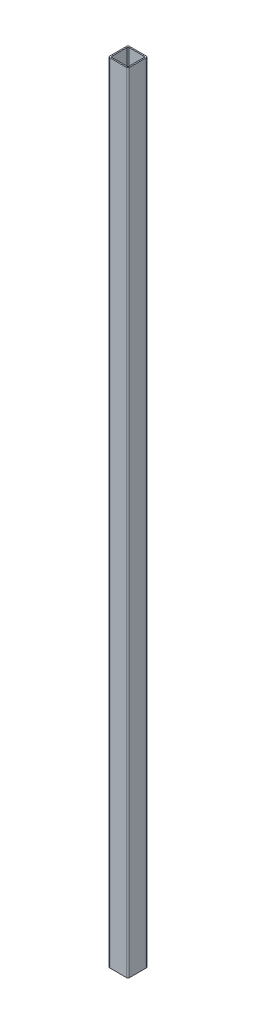
SolidWorks part; units mm, degrees
material "Angle steel 100×100×6/Q235"
ref_plane "Front Plane" through (0, 0, 0) normal (0, 0, 1) x (1, 0, 0)
ref_plane "Top Plane" through (0, 0, 0) normal (0, 1, 0) x (1, 0, 0)
ref_plane "Right Plane" through (0, 0, 0) normal (1, 0, 0) x (0, 0, -1)
sketch "Sketch2" plane through (0, 0, 0) normal (0, 1, 0) x (1, 0, 0)
  line L0 (12.6, 4.775) -> (87.4, 4.775)
  line L1 (6.3, 11.075) -> (6.3, 85.875)
  line L2 (87.4, 92.175) -> (12.6, 92.175)
  line L3 (93.7, 85.875) -> (93.7, 11.075)
  line L4 (7.875, -1.525) -> (92.125, -1.525)
  line L5 (0, 6.35) -> (0, 90.6)
  line L6 (92.125, 98.475) -> (7.875, 98.475)
  line L7 (100, 90.6) -> (100, 6.35)
  arc A0 (100, 90.6) -> (92.125, 98.475) centre (92.125, 90.6) ccw
  arc A1 (92.125, -1.525) -> (100, 6.35) centre (92.125, 6.35) ccw
  arc A2 (0, 6.35) -> (7.875, -1.525) centre (7.875, 6.35) ccw
  arc A3 (7.875, 98.475) -> (0, 90.6) centre (7.875, 90.6) ccw
  arc A4 (12.6, 92.175) -> (6.3, 85.875) centre (12.6, 85.875) ccw
  arc A5 (93.7, 85.875) -> (87.4, 92.175) centre (87.4, 85.875) ccw
  arc A6 (87.4, 4.775) -> (93.7, 11.075) centre (87.4, 11.075) ccw
  arc A7 (6.3, 11.075) -> (12.6, 4.775) centre (12.6, 11.075) ccw
extrude "Boss-Extrude1" add sketch "Sketch2" along normal mid plane 4000
